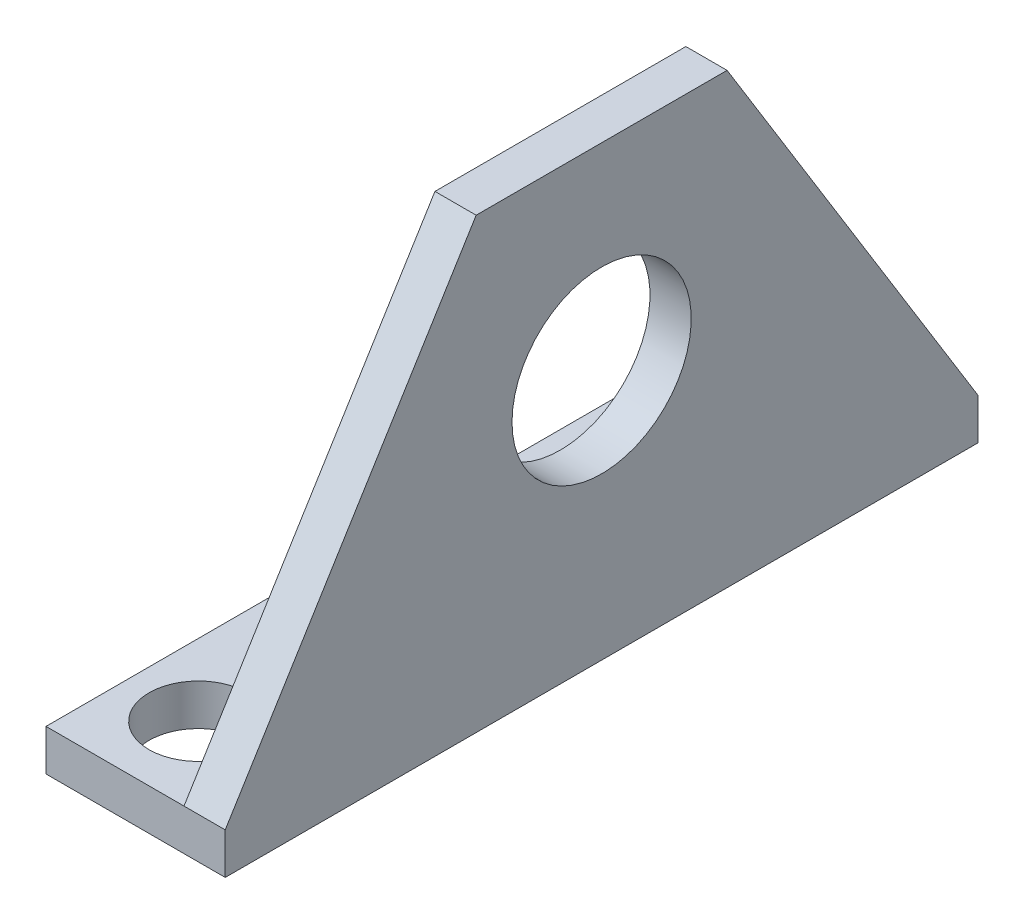
from build123d import *

# Parameters (mm, degrees)
BOSS_EXTRUDE1_DEPTH        = 2.3
SKETCH2_W                  = 42
SKETCH2_H                  = 2.3
BOSS_EXTRUDE2_DEPTH        = 7.7
F_10_0_10_DIAMETER_HOLE1_D = 10
F_5_5_5_5_DIAMETER_HOLE1_D = 5.5
CHAMFER1_SIZE              = 13.335010311


with BuildPart() as part:
    # Sketch1 → Boss-Extrude1 (new body)
    with BuildSketch(Plane(origin=(-2.3, 0, 0), x_dir=(0, -1, 0), z_dir=(-1, 0, 0))):
        Polygon((11.7, 21), (-22.35, 0), (11.7, -21), (14, -21), (14, 21), align=None)
    extrude(amount=-BOSS_EXTRUDE1_DEPTH)

    # Sketch2 → Boss-Extrude2 (add)
    with BuildSketch(Plane.ZY.offset(2.3)):
        with Locations((0, -12.85)):
            Rectangle(SKETCH2_W, SKETCH2_H)
    extrude(amount=BOSS_EXTRUDE2_DEPTH)

    # Ø10.0 (10) Diameter Hole1 (through all)
    with Locations(Plane.ZY.offset(2.3)):
        with Locations((0, 0)):
            Hole(F_10_0_10_DIAMETER_HOLE1_D / 2)

    # Ø5.5 (5.5) Diameter Hole1 (through all)
    with Locations(Plane(origin=(0, -11.7, 0), x_dir=(1, 0, 0), z_dir=(0, 1, 0))):
        with Locations((-6, -16.5), (-6, 16.5)):
            Hole(F_5_5_5_5_DIAMETER_HOLE1_D / 2)

    # Chamfer1
    chamfer1_edges = [part.edges().sort_by_distance(p)[0] for p in [
        (-1.15, 22.35, 0),
    ]]
    chamfer(chamfer1_edges, length=CHAMFER1_SIZE)


solid = part.part
